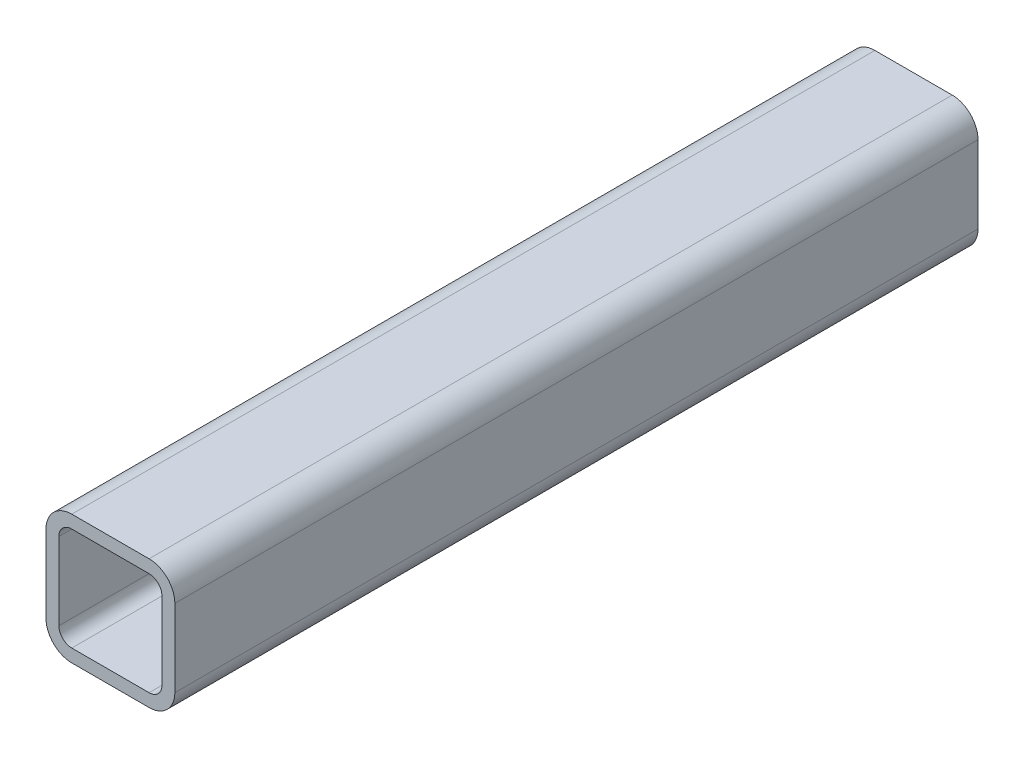
SolidWorks part; units mm, degrees
material "Q235B"
ref_plane "Plane1" through (0, 0, 0) normal (0, 0, 1) x (1, 0, 0)
ref_plane "Plane2" through (0, 0, 0) normal (0, 1, 0) x (1, 0, 0)
ref_plane "Plane3" through (0, 0, 0) normal (1, 0, 0) x (0, 0, -1)
sketch "Sketch1" plane through (0, 0, 0) normal (0, 0, 1) x (1, 0, 0)
  line L0 (-9, -12) -> (9, -12)
  line L1 (-12, -9) -> (-12, 9)
  line L2 (9, 12) -> (-9, 12)
  line L3 (12, 9) -> (12, -9)
  line L4 (-9, -15) -> (9, -15)
  line L5 (-15, -9) -> (-15, 9)
  line L6 (9, 15) -> (-9, 15)
  line L7 (15, 9) -> (15, -9)
  arc A0 (15, 9) -> (9, 15) centre (9, 9) ccw
  arc A1 (9, -15) -> (15, -9) centre (9, -9) ccw
  arc A2 (-15, -9) -> (-9, -15) centre (-9, -9) ccw
  arc A3 (-9, 15) -> (-15, 9) centre (-9, 9) ccw
  arc A4 (-9, 12) -> (-12, 9) centre (-9, 9) ccw
  arc A5 (12, 9) -> (9, 12) centre (9, 9) ccw
  arc A6 (9, -12) -> (12, -9) centre (9, -9) ccw
  arc A7 (-12, -9) -> (-9, -12) centre (-9, -9) ccw
  point P0 (-15, 0)
  point P1 (15, 0)
  point P2 (0, 15)
  point P3 (0, -15)
  point P4 (0, 0)
  point P5 (-15, -15)
  point P6 (15, -15)
  point P7 (15, 15)
  point P8 (-15, 15)
extrude "Boss-Extrude1" add sketch "Sketch1" along normal blind 187 contours L5 A3 L6 A0 L7 A1 L4 A2 | L1 A4 L2 A5 L3 A6 L0 A7
